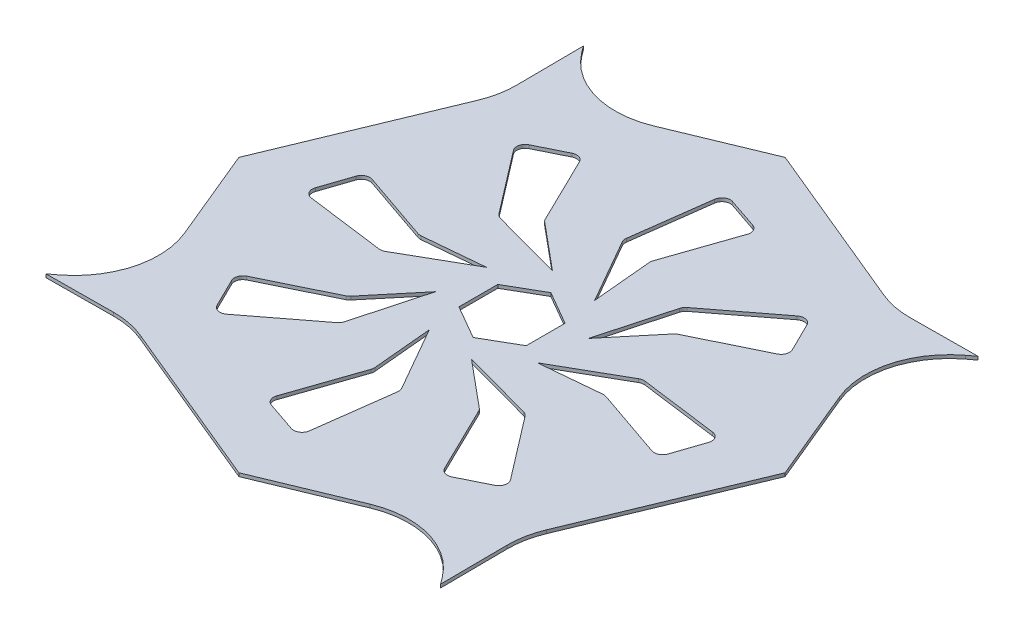
from build123d import *

# Parameters (mm, degrees)
BOSS_EXTRUDE1_DEPTH = 2
CUT_EXTRUDE1_DEPTH  = 10
CUT_EXTRUDE2_DEPTH  = 10
BOSS_EXTRUDE2_DEPTH = 2
FILLET1_R           = 50


with BuildPart() as part:
    # Sketch1 → Boss-Extrude1 (new body)
    with BuildSketch(Plane(origin=(0, 0, 0), x_dir=(1, 0, 0), z_dir=(0, 1, 0))):
        Polygon((114.80502971, -114.80502971), (162.358830044, 0), (114.80502971, 114.80502971), (0, 162.358830044), (-114.80502971, 114.80502971), (-162.358830044, 0), (-114.80502971, -114.80502971), (0, -162.358830044), align=None)
    extrude(amount=BOSS_EXTRUDE1_DEPTH)

    # Sketch2 → Cut-Extrude1 (cut)
    with BuildSketch(Plane(origin=(0, 2, 0), x_dir=(1, 0, 0), z_dir=(0, 1, 0))):
        Polygon((20, 11.547005384), (0, 23.094010768), (-20, 11.547005384), (-20, -11.547005384), (0, -23.094010768), (20, -11.547005384), align=None)
    extrude(amount=-CUT_EXTRUDE1_DEPTH, mode=Mode.SUBTRACT)

    # Sketch3 → Cut-Extrude2 (cut)
    with BuildSketch(Plane(origin=(0, 2, 0), x_dir=(1, 0, 0), z_dir=(0, 1, 0))):
        with BuildLine():
            Line((7.180747689, 123.974968015), (25.207285, 117.858821427))
            ThreePointArc((25.207285, 117.858821427), (28.089576698, 115.326406795), (28.328747659, 111.497108353))
            Line((28.328747659, 111.497108353), (13.99872444, 69.850478373))
            ThreePointArc((13.99872444, 69.850478373), (13.762569524, 68.82175425), (13.747623306, 67.766377979))
            Line((13.747623306, 67.766377979), (17.02042887, 32.130840461))
            Line((17.02042887, 32.130840461), (-4.884764675, 70.429589412))
            ThreePointArc((-4.884764675, 70.429589412), (-5.450629901, 71.947522663), (-5.501487679, 73.566700941))
            Line((-5.501487679, 73.566700941), (0.617313414, 119.89476636))
            ThreePointArc((0.617313414, 119.89476636), (2.934488498, 123.486434711), (7.180747689, 123.974968015))
        make_face()
        with BuildLine():
            Line((92.741095966, 82.585985196), (101.163014013, 65.514529695))
            ThreePointArc((101.163014013, 65.514529695), (101.410414459, 61.68575413), (98.871810971, 58.808911827))
            Line((98.871810971, 58.808911827), (59.290339906, 39.493153947))
            ThreePointArc((59.290339906, 39.493153947), (58.395935361, 38.932722886), (57.63910307, 38.197027741))
            Line((57.63910307, 38.197027741), (34.755195848, 10.684674503))
            Line((34.755195848, 10.684674503), (46.347190043, 53.255290495))
            ThreePointArc((46.347190043, 53.255290495), (47.0204038, 54.72875853), (48.129373861, 55.909652349))
            Line((48.129373861, 55.909652349), (85.214908823, 84.34189582))
            ThreePointArc((85.214908823, 84.34189582), (89.393092084, 85.243098653), (92.741095966, 82.585985196))
        make_face()
        with BuildLine():
            Line((123.974968015, -7.180747689), (117.858821427, -25.207285))
            ThreePointArc((117.858821427, -25.207285), (115.326406795, -28.089576698), (111.497108353, -28.328747659))
            Line((111.497108353, -28.328747659), (69.850478373, -13.99872444))
            ThreePointArc((69.850478373, -13.99872444), (68.82175425, -13.762569524), (67.766377979, -13.747623306))
            Line((67.766377979, -13.747623306), (32.130840461, -17.02042887))
            Line((32.130840461, -17.02042887), (70.429589412, 4.884764675))
            ThreePointArc((70.429589412, 4.884764675), (71.947522663, 5.450629901), (73.566700941, 5.501487679))
            Line((73.566700941, 5.501487679), (119.89476636, -0.617313414))
            ThreePointArc((119.89476636, -0.617313414), (123.486434711, -2.934488498), (123.974968015, -7.180747689))
        make_face()
        with BuildLine():
            Line((82.585985196, -92.741095966), (65.514529695, -101.163014013))
            ThreePointArc((65.514529695, -101.163014013), (61.68575413, -101.410414459), (58.808911827, -98.871810971))
            Line((58.808911827, -98.871810971), (39.493153947, -59.290339906))
            ThreePointArc((39.493153947, -59.290339906), (38.932722886, -58.395935361), (38.197027741, -57.63910307))
            Line((38.197027741, -57.63910307), (10.684674503, -34.755195848))
            Line((10.684674503, -34.755195848), (53.255290495, -46.347190043))
            ThreePointArc((53.255290495, -46.347190043), (54.72875853, -47.0204038), (55.909652349, -48.129373861))
            Line((55.909652349, -48.129373861), (84.34189582, -85.214908823))
            ThreePointArc((84.34189582, -85.214908823), (85.243098653, -89.393092084), (82.585985196, -92.741095966))
        make_face()
        with BuildLine():
            Line((-7.180747689, -123.974968015), (-25.207285, -117.858821427))
            ThreePointArc((-25.207285, -117.858821427), (-28.089576698, -115.326406795), (-28.328747659, -111.497108353))
            Line((-28.328747659, -111.497108353), (-13.99872444, -69.850478373))
            ThreePointArc((-13.99872444, -69.850478373), (-13.762569524, -68.82175425), (-13.747623306, -67.766377979))
            Line((-13.747623306, -67.766377979), (-17.02042887, -32.130840461))
            Line((-17.02042887, -32.130840461), (4.884764675, -70.429589412))
            ThreePointArc((4.884764675, -70.429589412), (5.450629901, -71.947522663), (5.501487679, -73.566700941))
            Line((5.501487679, -73.566700941), (-0.617313414, -119.89476636))
            ThreePointArc((-0.617313414, -119.89476636), (-2.934488497, -123.486434711), (-7.180747689, -123.974968015))
        make_face()
        with BuildLine():
            Line((-92.741095966, -82.585985196), (-101.163014013, -65.514529695))
            ThreePointArc((-101.163014013, -65.514529695), (-101.410414459, -61.68575413), (-98.871810971, -58.808911827))
            Line((-98.871810971, -58.808911827), (-59.290339906, -39.493153947))
            ThreePointArc((-59.290339906, -39.493153947), (-58.395935361, -38.932722886), (-57.63910307, -38.197027741))
            Line((-57.63910307, -38.197027741), (-34.755195848, -10.684674503))
            Line((-34.755195848, -10.684674503), (-46.347190043, -53.255290495))
            ThreePointArc((-46.347190043, -53.255290495), (-47.0204038, -54.72875853), (-48.129373861, -55.909652349))
            Line((-48.129373861, -55.909652349), (-85.214908823, -84.34189582))
            ThreePointArc((-85.214908823, -84.34189582), (-89.393092084, -85.243098653), (-92.741095966, -82.585985196))
        make_face()
        with BuildLine():
            Line((-123.974968015, 7.180747689), (-117.858821427, 25.207285))
            ThreePointArc((-117.858821427, 25.207285), (-115.326406795, 28.089576698), (-111.497108353, 28.328747659))
            Line((-111.497108353, 28.328747659), (-69.850478373, 13.99872444))
            ThreePointArc((-69.850478373, 13.99872444), (-68.82175425, 13.762569524), (-67.766377979, 13.747623306))
            Line((-67.766377979, 13.747623306), (-32.130840461, 17.02042887))
            Line((-32.130840461, 17.02042887), (-70.429589412, -4.884764675))
            ThreePointArc((-70.429589412, -4.884764675), (-71.947522663, -5.450629901), (-73.566700941, -5.501487679))
            Line((-73.566700941, -5.501487679), (-119.89476636, 0.617313414))
            ThreePointArc((-119.89476636, 0.617313414), (-123.486434711, 2.934488497), (-123.974968015, 7.180747689))
        make_face()
        with BuildLine():
            Line((-82.585985196, 92.741095966), (-65.514529695, 101.163014013))
            ThreePointArc((-65.514529695, 101.163014013), (-61.68575413, 101.410414459), (-58.808911827, 98.871810971))
            Line((-58.808911827, 98.871810971), (-39.493153947, 59.290339906))
            ThreePointArc((-39.493153947, 59.290339906), (-38.932722886, 58.395935361), (-38.197027741, 57.63910307))
            Line((-38.197027741, 57.63910307), (-10.684674503, 34.755195848))
            Line((-10.684674503, 34.755195848), (-53.255290495, 46.347190043))
            ThreePointArc((-53.255290495, 46.347190043), (-54.72875853, 47.0204038), (-55.909652349, 48.129373861))
            Line((-55.909652349, 48.129373861), (-84.34189582, 85.214908823))
            ThreePointArc((-84.34189582, 85.214908823), (-85.243098653, 89.393092084), (-82.585985196, 92.741095966))
        make_face()
    extrude(amount=-CUT_EXTRUDE2_DEPTH, mode=Mode.SUBTRACT)

    # Sketch6 → Boss-Extrude2 (add)
    with BuildSketch(Plane(origin=(0, 2, 0), x_dir=(1, 0, 0), z_dir=(0, 1, 0))):
        Polygon((-116.910273848, 109.722520758), (-117.296113887, 159.722520758), (-90.835857438, 124.733385943), (-114.80502971, 114.80502971), align=None)
        Polygon((109.722520758, 116.910273848), (159.722520758, 117.296113887), (124.733385943, 90.835857438), (114.80502971, 114.80502971), align=None)
        Polygon((116.910273848, -109.722520758), (117.296113887, -159.722520758), (90.835857438, -124.733385943), (114.80502971, -114.80502971), align=None)
        Polygon((-109.722520758, -116.910273848), (-159.722520758, -117.296113887), (-124.733385943, -90.835857438), (-114.80502971, -114.80502971), align=None)
    extrude(amount=-BOSS_EXTRUDE2_DEPTH)

    # Fillet1
    fillet1_edges = [part.edges().sort_by_distance(p)[0] for p in [
        (-116.910273848, 1, -109.722520758),
        (-90.835857438, 1, -124.733385943),
        (109.722520758, 1, -116.910273848),
        (124.733385943, 1, -90.835857438),
        (116.910273848, 1, 109.722520758),
        (90.835857438, 1, 124.733385943),
        (-109.722520758, 1, 116.910273848),
        (-124.733385943, 1, 90.835857438),
    ]]
    fillet(fillet1_edges, radius=FILLET1_R)


solid = part.part
